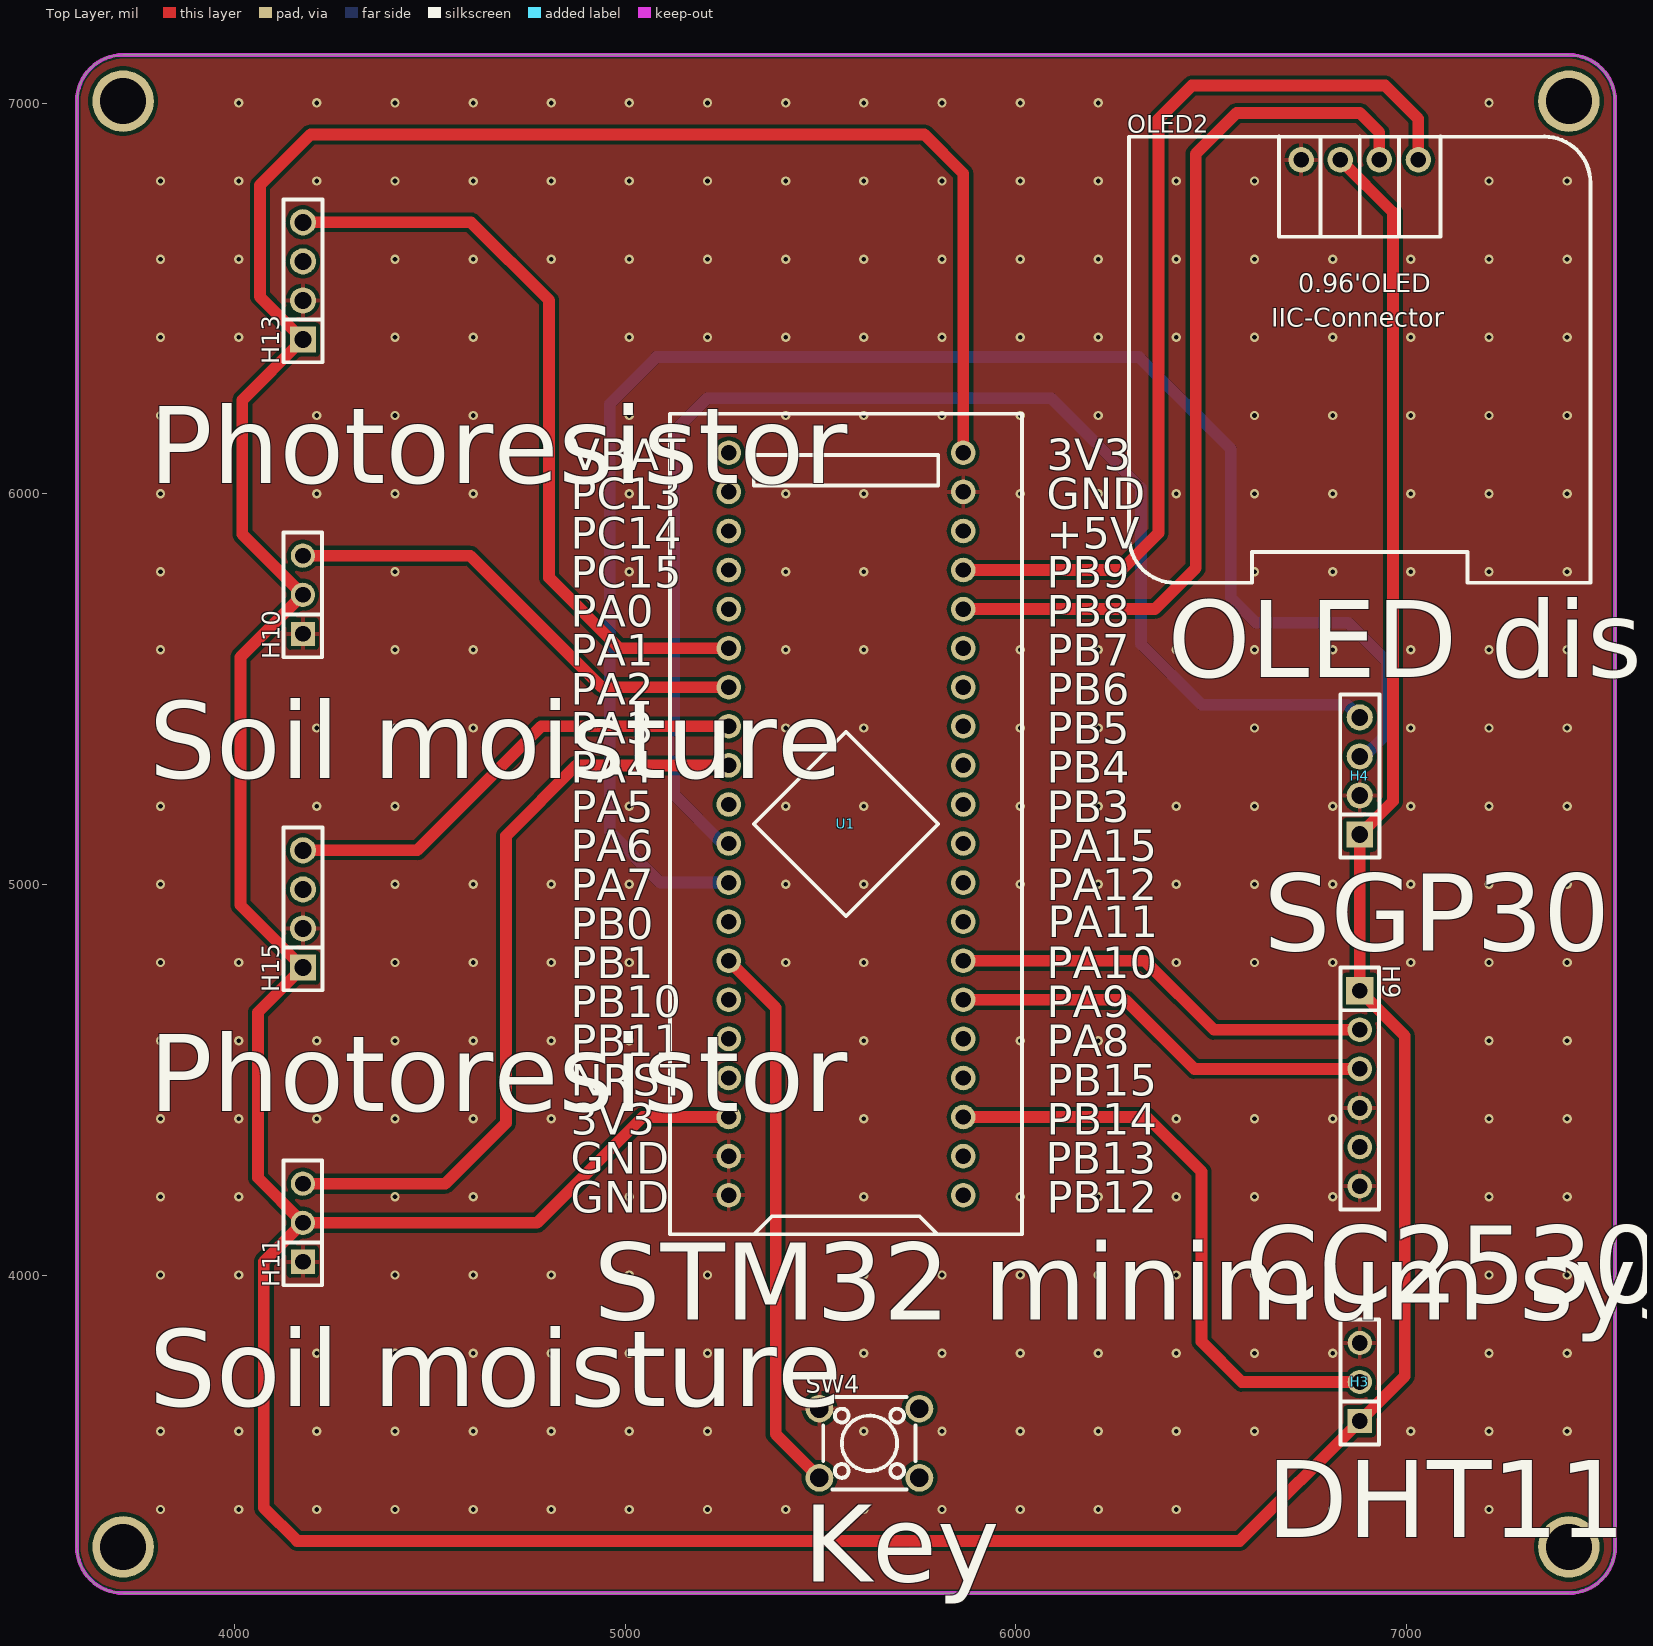
[diagram p0: Top Layer view]
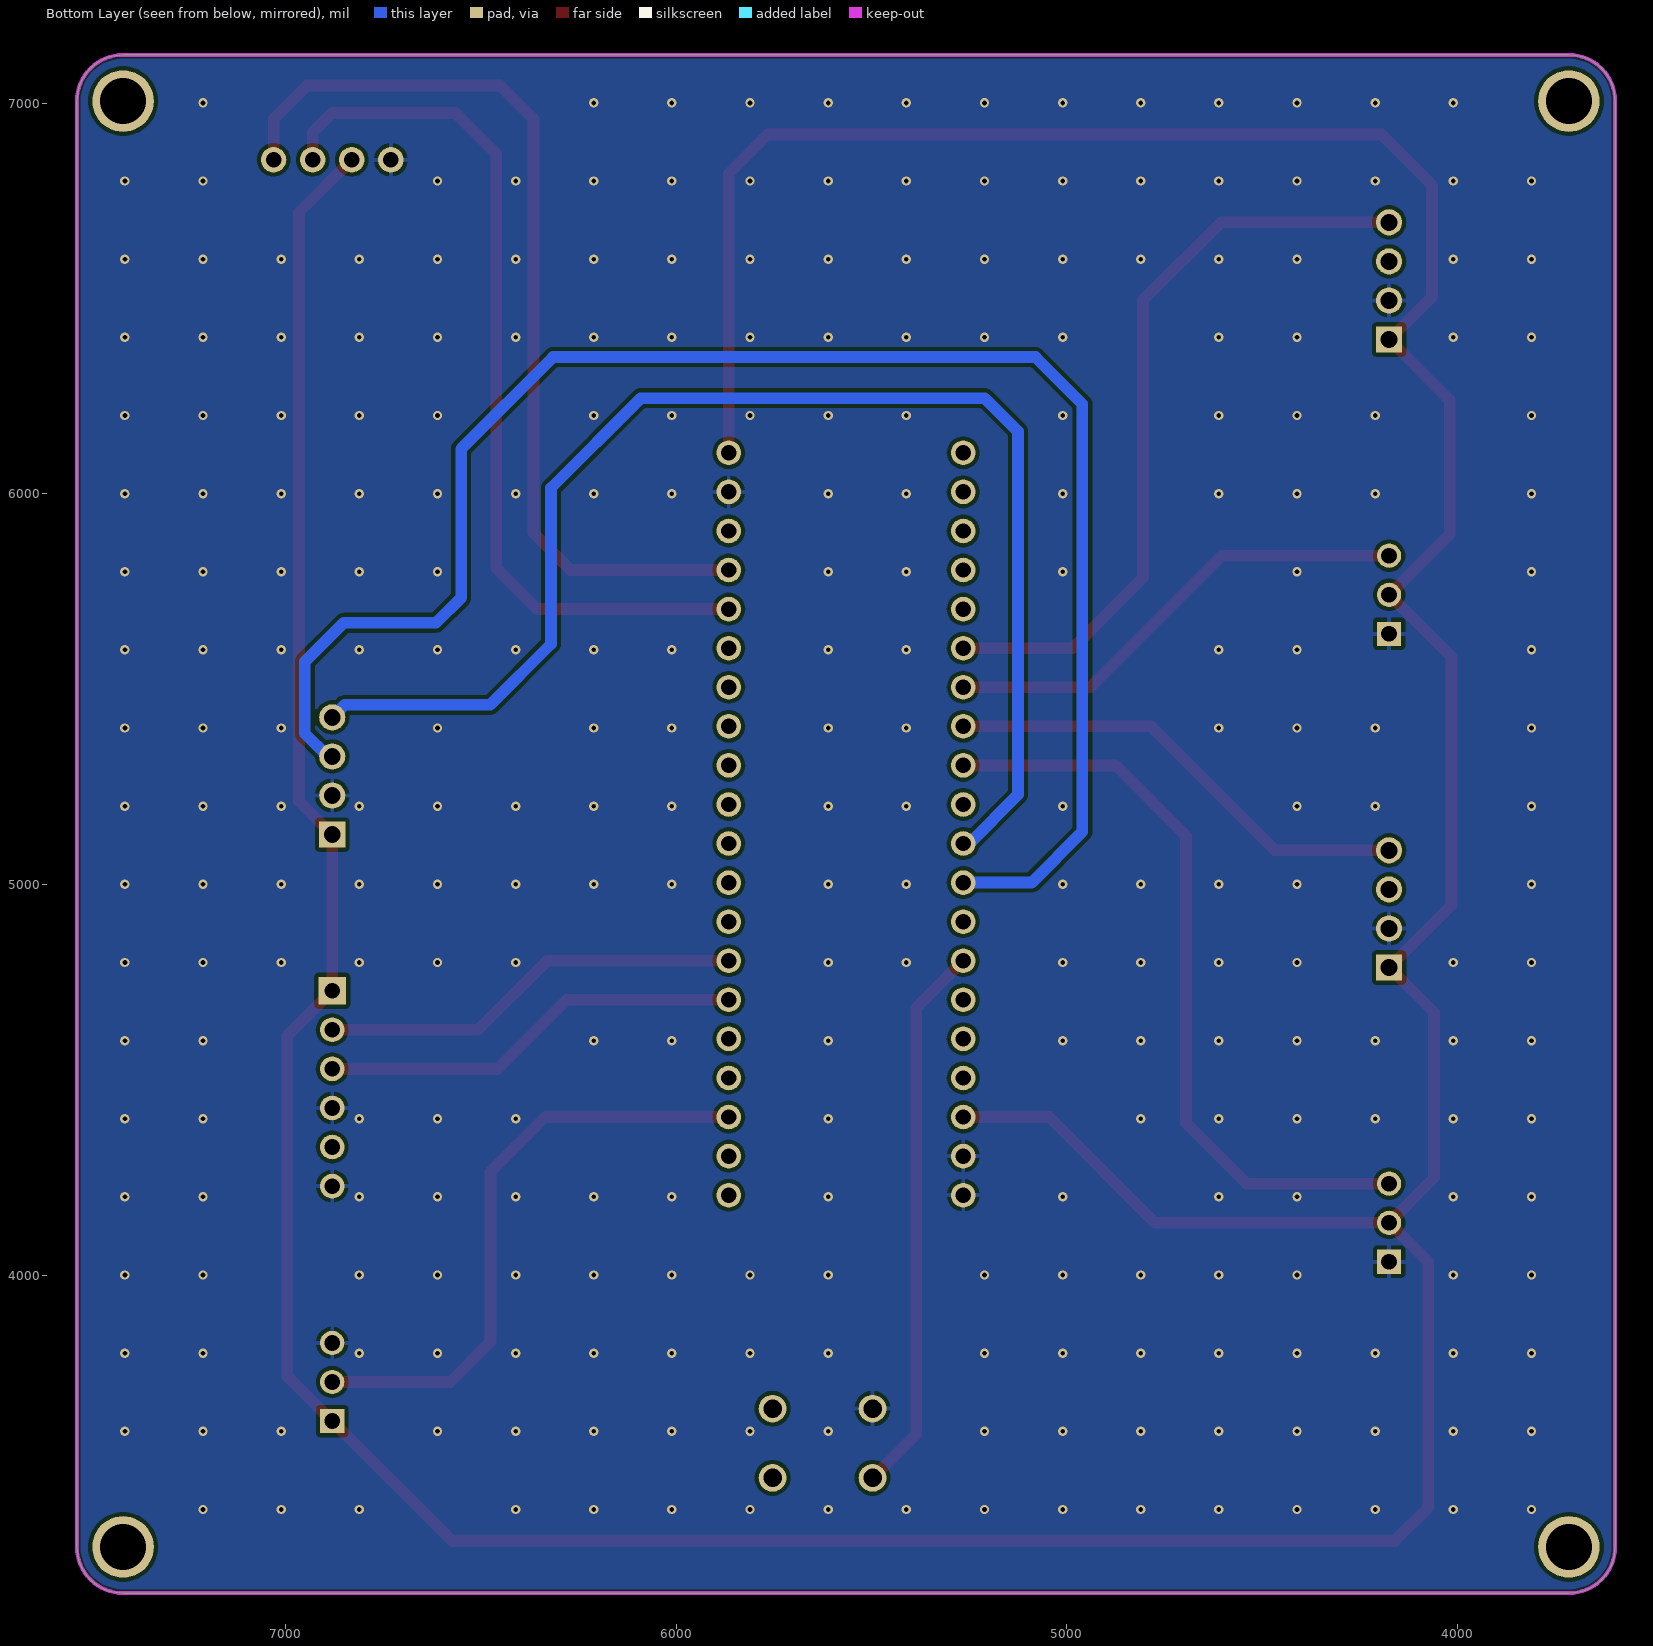
[diagram p1: Bottom Layer view, seen from below]
# Altium PCB MISC52023.pcbdoc
Units mil, origin at the board's own origin, x right, y up, seen from the top; angles counter-clockwise.
Board outline 3937.01 x 3937.01 mil, 2 copper layers (Top Layer, Bottom Layer), stack 62.206 mil thick; 10 components, 37 nets, 79 pads, 277 vias.

## Layer stack, top to bottom
Top Solder Mask Layer: solder mask 0.394, Dk 3.3
Top Layer: signal copper 1.379
Dielectric1: surface 59.449, FR4, Dk 4.5
Bottom Layer: signal copper 1.378
Bottom Solder Mask Layer: solder mask 0.394, Dk 3.3

## Board outline
3714.61,7123.5 ccw(c3714.61,7005.39) 3596.5,7005.39 3596.5,3304.61 ccw(c3714.61,3304.61) 3714.61,3186.5 7415.39,3186.5 ccw(c7415.39,3304.61) 7533.5,3304.61 7533.5,7005.39 ccw(c7415.39,7005.39) 7415.39,7123.5 3714.61,7123.5

## Design rules (kind name [scope] priority, off if disabled: settings)
BoardOutlineClearance copperThickness2oz_1 [All] p2 off: genericclearance=7.99 ignorepadtopadclearanceinfootprint=FALSE except(0: Arc-SplitContinuation Track-SplitContinuation SMDPad-SplitContinuation THPad-SplitContinuation Via-SplitContinuation Fill-SplitContinuation Region-SplitContinuation Poly-SplitContinuation Text-SplitContinuation Hole-SplitContinuation; 5.98: Arc-CutoutEdge Track-CutoutEdge SMDPad-CutoutEdge THPad-CutoutEdge Via-CutoutEdge Text-CutoutEdge; 6.9: Hole-OutlineEdge Hole-CutoutEdge; 10: Poly-OutlineEdge Poly-CutoutEdge; 11.81: Arc-OutlineEdge Track-OutlineEdge SMDPad-OutlineEdge THPad-OutlineEdge Via-OutlineEdge Fill-OutlineEdge Region-OutlineEdge Text-OutlineEdge Fill-CutoutEdge Region-CutoutEdge)
BoardOutlineClearance Plane_innerPlane_1 [All] p4 off: genericclearance=4.02 ignorepadtopadclearanceinfootprint=FALSE except(0: Arc-SplitContinuation Track-SplitContinuation SMDPad-SplitContinuation THPad-SplitContinuation Via-SplitContinuation Fill-SplitContinuation Region-SplitContinuation Poly-SplitContinuation Text-SplitContinuation Hole-SplitContinuation; 5.98: Arc-CutoutEdge Track-CutoutEdge SMDPad-CutoutEdge THPad-CutoutEdge Via-CutoutEdge Text-CutoutEdge; 6.9: Hole-OutlineEdge Hole-CutoutEdge; 10: Poly-OutlineEdge Poly-CutoutEdge; 11.81: Arc-OutlineEdge Track-OutlineEdge SMDPad-OutlineEdge THPad-OutlineEdge Via-OutlineEdge Fill-OutlineEdge Region-OutlineEdge Text-OutlineEdge Fill-CutoutEdge Region-CutoutEdge)
BoardOutlineClearance Copper_copperRegion_1 [All] p6 off: genericclearance=4.02 ignorepadtopadclearanceinfootprint=FALSE except(0: Arc-SplitContinuation Track-SplitContinuation SMDPad-SplitContinuation THPad-SplitContinuation Via-SplitContinuation Fill-SplitContinuation Region-SplitContinuation Poly-SplitContinuation Text-SplitContinuation Hole-SplitContinuation; 5.98: Arc-CutoutEdge Track-CutoutEdge SMDPad-CutoutEdge THPad-CutoutEdge Via-CutoutEdge Text-CutoutEdge; 6.9: Hole-OutlineEdge Hole-CutoutEdge; 10: Poly-OutlineEdge Poly-CutoutEdge; 11.81: Arc-OutlineEdge Track-OutlineEdge SMDPad-OutlineEdge THPad-OutlineEdge Via-OutlineEdge Fill-OutlineEdge Region-OutlineEdge Text-OutlineEdge Fill-CutoutEdge Region-CutoutEdge)
BoardOutlineClearance Copper_copperRegion_copperThickness1oz_1 [All] p8 off: genericclearance=4.02 ignorepadtopadclearanceinfootprint=FALSE except(0: Arc-SplitContinuation Track-SplitContinuation SMDPad-SplitContinuation THPad-SplitContinuation Via-SplitContinuation Fill-SplitContinuation Region-SplitContinuation Poly-SplitContinuation Text-SplitContinuation Hole-SplitContinuation; 5.98: Arc-CutoutEdge Track-CutoutEdge SMDPad-CutoutEdge THPad-CutoutEdge Via-CutoutEdge Text-CutoutEdge; 6.9: Hole-OutlineEdge Hole-CutoutEdge; 10: Poly-OutlineEdge Poly-CutoutEdge; 11.81: Arc-OutlineEdge Track-OutlineEdge SMDPad-OutlineEdge THPad-OutlineEdge Via-OutlineEdge Fill-OutlineEdge Region-OutlineEdge Text-OutlineEdge Fill-CutoutEdge Region-CutoutEdge)
BoardOutlineClearance Copper_copperRegion_Copper_copperRegion_1 [All] p10 off: genericclearance=4.02 ignorepadtopadclearanceinfootprint=FALSE except(0: Arc-SplitContinuation Track-SplitContinuation SMDPad-SplitContinuation THPad-SplitContinuation Via-SplitContinuation Fill-SplitContinuation Region-SplitContinuation Poly-SplitContinuation Text-SplitContinuation Hole-SplitContinuation; 5.98: Arc-CutoutEdge Track-CutoutEdge SMDPad-CutoutEdge THPad-CutoutEdge Via-CutoutEdge Text-CutoutEdge; 6.9: Hole-OutlineEdge Hole-CutoutEdge; 10: Poly-OutlineEdge Poly-CutoutEdge; 11.81: Arc-OutlineEdge Track-OutlineEdge SMDPad-OutlineEdge THPad-OutlineEdge Via-OutlineEdge Fill-OutlineEdge Region-OutlineEdge Text-OutlineEdge Fill-CutoutEdge Region-CutoutEdge)
BoardOutlineClearance copperThickness1oz_1 [All] p12: genericclearance=4.02 ignorepadtopadclearanceinfootprint=FALSE except(0: Arc-SplitContinuation Track-SplitContinuation SMDPad-SplitContinuation THPad-SplitContinuation Via-SplitContinuation Fill-SplitContinuation Region-SplitContinuation Poly-SplitContinuation Text-SplitContinuation Hole-SplitContinuation; 5.98: Arc-CutoutEdge Track-CutoutEdge SMDPad-CutoutEdge THPad-CutoutEdge Via-CutoutEdge Text-CutoutEdge; 6.9: Hole-OutlineEdge Hole-CutoutEdge; 10: Poly-OutlineEdge Poly-CutoutEdge; 11.81: Arc-OutlineEdge Track-OutlineEdge SMDPad-OutlineEdge THPad-OutlineEdge Via-OutlineEdge Fill-OutlineEdge Region-OutlineEdge Text-OutlineEdge Fill-CutoutEdge Region-CutoutEdge)
Clearance copperThickness2oz [All] p1 off: gap=7.99 ignorepadtopadclearanceinfootprint=FALSE except(5.98: SMDPad-Track SMDPad-SMDPad THPad-Track SMDPad-THPad THPad-THPad Track-Via SMDPad-Via THPad-Via Via-Via Fill-SMDPad Region-SMDPad Fill-THPad Region-THPad Fill-Via Region-Via Fill-Fill Fill-Region Region-Region Arc-Track Arc-SMDPad Arc-THPad Arc-Via Fill-Arc Region-Arc Arc-Arc Text-Track SMDPad-Text Text-THPad Text-Via Fill-Text Region-Text Arc-Text Text-Text; 6.9: Hole-Track Hole-SMDPad Hole-THPad Hole-Via Fill-Hole Region-Hole Hole-Arc Hole-Text; 10: Poly-Track Poly-SMDPad Poly-THPad Poly-Via Poly-Fill Poly-Region Poly-Poly Poly-Arc Poly-Text Poly-Hole; 11.81: Fill-Track Region-Track)
Clearance Plane_innerPlane [All] p3 off: gap=4.02 ignorepadtopadclearanceinfootprint=FALSE except(5.98: SMDPad-Track SMDPad-SMDPad THPad-Track SMDPad-THPad THPad-THPad Track-Via SMDPad-Via THPad-Via Via-Via Fill-SMDPad Region-SMDPad Fill-THPad Region-THPad Fill-Via Region-Via Fill-Fill Fill-Region Region-Region Arc-Track Arc-SMDPad Arc-THPad Arc-Via Fill-Arc Region-Arc Arc-Arc Text-Track SMDPad-Text Text-THPad Text-Via Fill-Text Region-Text Arc-Text Text-Text; 6.9: Hole-Track Hole-SMDPad Hole-THPad Hole-Via Fill-Hole Region-Hole Hole-Arc Hole-Text; 10: Poly-Track Poly-SMDPad Poly-THPad Poly-Via Poly-Fill Poly-Region Poly-Poly Poly-Arc Poly-Text Poly-Hole; 11.81: Fill-Track Region-Track)
Clearance Copper_copperRegion [All] p5 off: gap=4.02 ignorepadtopadclearanceinfootprint=FALSE except(5.98: SMDPad-Track SMDPad-SMDPad THPad-Track SMDPad-THPad THPad-THPad Track-Via SMDPad-Via THPad-Via Via-Via Fill-SMDPad Region-SMDPad Fill-THPad Region-THPad Fill-Via Region-Via Fill-Fill Fill-Region Region-Region Arc-Track Arc-SMDPad Arc-THPad Arc-Via Fill-Arc Region-Arc Arc-Arc Text-Track SMDPad-Text Text-THPad Text-Via Fill-Text Region-Text Arc-Text Text-Text; 6.9: Hole-Track Hole-SMDPad Hole-THPad Hole-Via Fill-Hole Region-Hole Hole-Arc Hole-Text; 10: Poly-Track Poly-SMDPad Poly-THPad Poly-Via Poly-Fill Poly-Region Poly-Poly Poly-Arc Poly-Text Poly-Hole; 11.81: Fill-Track Region-Track)
Clearance Copper_copperRegion_copperThickness1oz [All] p7 off: gap=4.02 ignorepadtopadclearanceinfootprint=FALSE except(5.98: SMDPad-Track SMDPad-SMDPad THPad-Track SMDPad-THPad THPad-THPad Track-Via SMDPad-Via THPad-Via Via-Via Fill-SMDPad Region-SMDPad Fill-THPad Region-THPad Fill-Via Region-Via Fill-Fill Fill-Region Region-Region Arc-Track Arc-SMDPad Arc-THPad Arc-Via Fill-Arc Region-Arc Arc-Arc Text-Track SMDPad-Text Text-THPad Text-Via Fill-Text Region-Text Arc-Text Text-Text; 6.9: Hole-Track Hole-SMDPad Hole-THPad Hole-Via Fill-Hole Region-Hole Hole-Arc Hole-Text; 10: Poly-Track Poly-SMDPad Poly-THPad Poly-Via Poly-Fill Poly-Region Poly-Poly Poly-Arc Poly-Text Poly-Hole; 11.81: Fill-Track Region-Track)
Clearance Copper_copperRegion_Copper_copperRegion [All] p9 off: gap=4.02 ignorepadtopadclearanceinfootprint=FALSE except(5.98: SMDPad-Track SMDPad-SMDPad THPad-Track SMDPad-THPad THPad-THPad Track-Via SMDPad-Via THPad-Via Via-Via Fill-SMDPad Region-SMDPad Fill-THPad Region-THPad Fill-Via Region-Via Fill-Fill Fill-Region Region-Region Arc-Track Arc-SMDPad Arc-THPad Arc-Via Fill-Arc Region-Arc Arc-Arc Text-Track SMDPad-Text Text-THPad Text-Via Fill-Text Region-Text Arc-Text Text-Text; 6.9: Hole-Track Hole-SMDPad Hole-THPad Hole-Via Fill-Hole Region-Hole Hole-Arc Hole-Text; 10: Poly-Track Poly-SMDPad Poly-THPad Poly-Via Poly-Fill Poly-Region Poly-Poly Poly-Arc Poly-Text Poly-Hole; 11.81: Fill-Track Region-Track)
Clearance copperThickness1oz [All] p11: gap=4.02 ignorepadtopadclearanceinfootprint=FALSE except(5.98: SMDPad-Track SMDPad-SMDPad THPad-Track SMDPad-THPad THPad-THPad Track-Via SMDPad-Via THPad-Via Via-Via Fill-SMDPad Region-SMDPad Fill-THPad Region-THPad Fill-Via Region-Via Fill-Fill Fill-Region Region-Region Arc-Track Arc-SMDPad Arc-THPad Arc-Via Fill-Arc Region-Arc Arc-Arc Text-Track SMDPad-Text Text-THPad Text-Via Fill-Text Region-Text Arc-Text Text-Text; 6.9: Hole-Track Hole-SMDPad Hole-THPad Hole-Via Fill-Hole Region-Hole Hole-Arc Hole-Text; 10: Poly-Track Poly-SMDPad Poly-THPad Poly-Via Poly-Fill Poly-Region Poly-Poly Poly-Arc Poly-Text Poly-Hole; 11.81: Fill-Track Region-Track)
DiffPairsRouting differentialPair [All] p1: maxlimit=6 minlimit=6 mostfreqgap=6 toplayer_minwidth=5 toplayer_prefwidth=10 toplayer_maxwidth=100 toplayer_mingap=6 toplayer_prefgap=6 toplayer_maxgap=6 bottomlayer_minwidth=5 bottomlayer_prefwidth=10 bottomlayer_maxwidth=100 bottomlayer_mingap=6 bottomlayer_prefgap=6 bottomlayer_maxgap=6 maxuncoupledlength=10
HoleToHoleClearance otherClearance [All] p1: gap=11.81 allowstackedmicrovias=TRUE
Length netLength [All] p1: minlimit=0 maxlimit=0
PasteMaskExpansion pasteMaskExpansion [All] p1: expansion=0
PlaneConnect innerPlane [All] p1: planeconnectstyle=Relief reliefexpansion=20 reliefentries=4 reliefconductorwidth=10 reliefairgap=10
PolygonConnect copperRegion_copperThickness1oz [All] p1 off: connectstyle=Relief reliefconductorwidth=10 reliefentries=4 polygonreliefangle="90 Angle" airgapwidth=10 via.connectstyle=Relief via.reliefconductorwidth=10 via.reliefentries=4 via.polygonreliefangle="90 Angle" via.airgapwidth=10
PolygonConnect copperRegion_Copper_copperRegion [All] p2 off: connectstyle=Relief reliefconductorwidth=10 reliefentries=4 polygonreliefangle="90 Angle" airgapwidth=10 via.connectstyle=Relief via.reliefconductorwidth=10 via.reliefentries=4 via.polygonreliefangle="90 Angle" via.airgapwidth=10
PolygonConnect copperRegion [All] p3: connectstyle=Relief reliefconductorwidth=10 reliefentries=4 polygonreliefangle="90 Angle" airgapwidth=10 via.connectstyle=Relief via.reliefconductorwidth=10 via.reliefentries=4 via.polygonreliefangle="90 Angle" via.airgapwidth=10
RoutingVias viaSize [All] p1: holewidth=12.01 width=24.02 viastyle="Through Hole" minholewidth=11.81 minwidth=19.68 maxholewidth=248.03 maxwidth=393.7
SolderMaskExpansion solderMaskExpansion [IsVia] p1: expansion=-1000 istentingtop=TRUE
SolderMaskExpansion solderMaskExpansion [All] p2: expansion=2 istentingtop=FALSE
Width copperThickness2oz_2 [All] p1 off: maxlimit=100 minlimit=8 preferedwidth=10
Width copperThickness1oz_2 [All] p2: maxlimit=100 minlimit=5 preferedwidth=10

## Components (designator, comment, footprint, x,y, rotation, side; value= is the part's Value field where it differs from the comment)
H3 "" HDR-TH_3P-P2.54-V-F 6880,3726.86 r90 top
H4 "" HDR-TH_4P-P2.54-V-F 6880,5277.96 r90 top
H9 "" HDR-TH_6P-P2.54-V-F 6880,4478.2 r270 top
H10 "" HDR-TH_3P-P2.54-V-F 4175,5741.64 r90 top
H11 "" HDR-TH_3P-P2.54-V-F 4175,4134.33 r90 top
H13 "" HDR-TH_4P-P2.54-V-F 4175,6545 r90 top
H15 "" HDR-TH_4P-P2.54-V-F 4175,4937.69 r90 top
OLED2 "" 0.96OLED_4P 6880,6855 r0 top
SW4 "" SW-TH_4P-L6.0-W6.0-P4.50-LS6.5 5625,3570 r0 top
U1 "STM32F103C8T6-Card" CONN-TH_L53.3-W22.9_STM32F103C8T6-CARD 5565,5155 r90 top

## Footprints (in the part's own frame and the unit in brackets; to place one, negate y for a bottom-side part, rotate by r counter-clockwise, add the part's x,y. Pads: shape width x height; smd on the part's side, far side on the other; paste and mask are expansions set on the pad)
0.96OLED_4P [mm]
  round 1.65 hole 1 copper offset 0,0: 1(-3.81,-0.001) 2(-1.27,0.002) 3(1.27,0.002) 4(3.81,0.002)
  silkscreen extent -15,-27.5 15,1.5
CONN-TH_L53.3-W22.9_STM32F103C8T6-CARD [mm]
  round 1.6 hole 1: 1(-24.13,-7.62) 2(-21.59,-7.62) 3(-19.05,-7.62) 4(-16.51,-7.62) 5(-13.97,-7.62) 6(-11.43,-7.62) 7(-8.89,-7.62) 8(-6.35,-7.62) 9(-3.81,-7.62) 10(-1.27,-7.62) 11(1.27,-7.62) 12(3.81,-7.62) 13(6.35,-7.62) 14(8.89,-7.62) 15(11.43,-7.62) 16(13.97,-7.62) 17(16.51,-7.62) 18(19.05,-7.62) 19(21.59,-7.62) 20(24.13,-7.62) 21(24.13,7.62) 22(21.59,7.62) 23(19.05,7.62) 24(16.51,7.62) 25(13.97,7.62) 26(11.43,7.62) 27(8.89,7.62) 28(6.35,7.62) 29(3.81,7.62) 30(1.27,7.62) 31(-1.27,7.62) 32(-3.81,7.62) 33(-6.35,7.62) 34(-8.89,7.62) 35(-11.43,7.62) 36(-13.97,7.62) 37(-16.51,7.62) 38(-19.05,7.62) 39(-21.59,7.62) 40(-24.13,7.62)
  silkscreen extent -26.67,-11.43 26.67,11.43
HDR-TH_3P-P2.54-V-F [mil]
  rect 62x62 hole 40.16: 1(-100,0)
  round 62 hole 40.16: 2(0,0) 3(100,0)
  silkscreen extent -160,-49 160,49
HDR-TH_4P-P2.54-V-F [mm]
  rect 1.7x1.7 hole 1.1: 1(-3.81,0)
  round 1.7 hole 1.1: 2(-1.27,0) 3(1.27,0) 4(3.81,0)
  silkscreen extent -5.29,-1.27 5.29,1.27
HDR-TH_6P-P2.54-V-F [mm]
  rect 1.8x1.8 hole 1.02: 1(-6.35,0)
  round 1.6 hole 1.02: 2(-3.81,0) 3(-1.27,0) 4(1.27,0) 5(3.81,0) 6(6.35,0)
  silkscreen extent -7.87,-1.25 7.87,1.25
SW-TH_4P-L6.0-W6.0-P4.50-LS6.5 [mm]
  round 1.8 hole 1.2: 1(-3.25,2.25) 2(3.25,2.25) 3(-3.25,-2.25) 4(3.25,-2.25)
  silkscreen extent -3,-3 3,3

## Free pads (board coordinates)
  round 157.48 hole 118.11: 1(3714.61,7005.39) 1(3714.61,3304.61) 1(7415.39,7005.39) 1(7415.39,3304.61)

## Via types
v1: diameter 24.02, hole 12, Top Layer to Bottom Layer, 277 vias

## Nets (pads, with @x,y where several pads share a name; then routed paths per layer and width w, separated by ;. In a path a pad name is that pad's centre, name@x,y a point inside that pad or via, vN(x,y) a via of type N, cw(c..) or ccw(c..) an arc to the next point about the centre after c; other vN are vias at no path point)
+5V: U1.18
GND: H3.3 H4.2 H9.4 H9.6 H10.1 H11.1 H13.2 H15.2 OLED2.1 SW4.1 U1.19 U1.39 U1.40
  other v1: 3810.6,3400.6 4010.6,3400.6 4210.6,3400.6 4410.6,3400.6 4610.6,3400.6 4810.6,3400.6 5010.6,3400.6 5210.6,3400.6 5410.6,3400.6 5610.6,3400.6 5810.6,3400.6 6010.6,3400.6 6210.6,3400.6 6410.6,3400.6 6810.6,3400.6 7010.6,3400.6 7210.6,3400.6 3810.6,3600.6 4010.6,3600.6 4210.6,3600.6 4410.6,3600.6 4610.6,3600.6 4810.6,3600.6 5010.6,3600.6 5210.6,3600.6 5610.6,3600.6 5810.6,3600.6 6010.6,3600.6 6210.6,3600.6 6410.6,3600.6 6610.6,3600.6 7010.6,3600.6 7210.6,3600.6 7410.6,3600.6 3810.6,3800.6 4010.6,3800.6 4210.6,3800.6 4410.6,3800.6 4610.6,3800.6 4810.6,3800.6 5010.6,3800.6 5210.6,3800.6 5610.6,3800.6 5810.6,3800.6 6010.6,3800.6 6210.6,3800.6 6410.6,3800.6 6610.6,3800.6 6810.6,3800.6 7210.6,3800.6 7410.6,3800.6 3810.6,4000.6 4010.6,4000.6 4410.6,4000.6 4610.6,4000.6 4810.6,4000.6 5010.6,4000.6 5210.6,4000.6 5610.6,4000.6 5810.6,4000.6 6010.6,4000.6 6210.6,4000.6 6410.6,4000.6 6610.6,4000.6 6810.6,4000.6 7210.6,4000.6 7410.6,4000.6 3810.6,4200.6 4010.6,4200.6 4410.6,4200.6 4610.6,4200.6 5010.6,4200.6 5610.6,4200.6 6010.6,4200.6 6210.6,4200.6 6410.6,4200.6 6610.6,4200.6 6810.6,4200.6 7210.6,4200.6 7410.6,4200.6 3810.6,4400.6 4010.6,4400.6 4210.6,4400.6 4410.6,4400.6 4610.6,4400.6 4810.6,4400.6 5610.6,4400.6 6410.6,4400.6 6610.6,4400.6 6810.6,4400.6 7210.6,4400.6 7410.6,4400.6 3810.6,4600.6 4010.6,4600.6 4210.6,4600.6 4410.6,4600.6 4610.6,4600.6 4810.6,4600.6 5010.6,4600.6 5610.6,4600.6 6010.6,4600.6 6210.6,4600.6 7210.6,4600.6 7410.6,4600.6 3810.6,4800.6 4010.6,4800.6 4410.6,4800.6 4610.6,4800.6 4810.6,4800.6 5010.6,4800.6 5410.6,4800.6 5610.6,4800.6 6410.6,4800.6 6610.6,4800.6 6810.6,4800.6 7010.6,4800.6 7210.6,4800.6 7410.6,4800.6 3810.6,5000.6 4410.6,5000.6 4610.6,5000.6 4810.6,5000.6 5010.6,5000.6 5410.6,5000.6 5610.6,5000.6 6010.6,5000.6 6210.6,5000.6 6410.6,5000.6 6610.6,5000.6 6810.6,5000.6 7010.6,5000.6 7210.6,5000.6 7410.6,5000.6 3810.6,5200.6 4210.6,5200.6 4410.6,5200.6 5010.6,5200.6 5410.6,5200.6 5610.6,5200.6 6010.6,5200.6 6210.6,5200.6 6410.6,5200.6 6610.6,5200.6 6810.6,5200.6 7010.6,5200.6 7210.6,5200.6 7410.6,5200.6 3810.6,5400.6 4210.6,5400.6 4410.6,5400.6 4610.6,5400.6 5410.6,5400.6 5610.6,5400.6 6010.6,5400.6 6210.6,5400.6 6610.6,5400.6 7010.6,5400.6 7210.6,5400.6 7410.6,5400.6 3810.6,5600.6 4410.6,5600.6 4610.6,5600.6 5410.6,5600.6 5610.6,5600.6 6010.6,5600.6 6210.6,5600.6 6410.6,5600.6 6610.6,5600.6 6810.6,5600.6 7010.6,5600.6 7210.6,5600.6 7410.6,5600.6 3810.6,5800.6 4410.6,5800.6 5010.6,5800.6 5410.6,5800.6 5610.6,5800.6 6610.6,5800.6 6810.6,5800.6 7010.6,5800.6 7210.6,5800.6 7410.6,5800.6 3810.6,6000.6 4210.6,6000.6 4410.6,6000.6 4610.6,6000.6 5010.6,6000.6 5410.6,6000.6 5610.6,6000.6 6010.6,6000.6 6210.6,6000.6 6410.6,6000.6 6610.6,6000.6 6810.6,6000.6 7010.6,6000.6 7210.6,6000.6 7410.6,6000.6 3810.6,6200.6 4210.6,6200.6 4410.6,6200.6 4610.6,6200.6 5010.6,6200.6 5410.6,6200.6 5610.6,6200.6 5810.6,6200.6 6010.6,6200.6 6210.6,6200.6 6610.6,6200.6 6810.6,6200.6 7010.6,6200.6 7210.6,6200.6 7410.6,6200.6 3810.6,6400.6 4010.6,6400.6 4410.6,6400.6 4610.6,6400.6 5010.6,6400.6 5210.6,6400.6 5410.6,6400.6 5610.6,6400.6 5810.6,6400.6 6010.6,6400.6 6210.6,6400.6 6410.6,6400.6 6610.6,6400.6 6810.6,6400.6 7010.6,6400.6 7210.6,6400.6 7410.6,6400.6 3810.6,6600.6 4010.6,6600.6 4410.6,6600.6 4610.6,6600.6 4810.6,6600.6 5010.6,6600.6 5210.6,6600.6 5410.6,6600.6 5610.6,6600.6 5810.6,6600.6 6010.6,6600.6 6210.6,6600.6 6410.6,6600.6 6610.6,6600.6 6810.6,6600.6 7010.6,6600.6 7210.6,6600.6 7410.6,6600.6 3810.6,6800.6 4010.6,6800.6 4210.6,6800.6 4410.6,6800.6 4610.6,6800.6 4810.6,6800.6 5010.6,6800.6 5210.6,6800.6 5410.6,6800.6 5610.6,6800.6 5810.6,6800.6 6010.6,6800.6 6210.6,6800.6 6410.6,6800.6 6610.6,6800.6 7210.6,6800.6 7410.6,6800.6 4010.6,7000.6 4210.6,7000.6 4410.6,7000.6 4610.6,7000.6 4810.6,7000.6 5010.6,7000.6 5210.6,7000.6 5410.6,7000.6 5610.6,7000.6 5810.6,7000.6 6010.6,7000.6 6210.6,7000.6 7210.6,7000.6
NRST: U1.37
PA0: U1.25
PA1: H13.4 U1.26 | length 1957.4
  Top Layer w30: H13.4 4605,6695 4805,6495 4805,5785 4985,5605 U1.26
PA2: H10.3 U1.27 | length 1229.4
  Top Layer w30: H10.3 4603.36,5841.64 4940,5505 U1.27
PA3: H15.4 U1.28 | length 1221.4
  Top Layer w30: H15.4 4467.69,5087.69 4785,5405 U1.28
PA4: H11.3 U1.29 | length 1964
  Top Layer w30: H11.3 4539.33,4234.33 4695,4390 4695,5125 4875,5305 U1.29
PA5: U1.30
PA6: H4.4 U1.31 | length 3484.3
  Bottom Layer w30: U1.31 5250,5105 5125,5230 5125,6160 5210,6245 6090,6245 6320,6015 6320,5615.65 6475.65,5460 6847.95,5460 H4.4
PA7: H4.3 U1.32 | length 4317.2
  Bottom Layer w30: U1.32 5090,5005 4960,5135 4960,6230 5080,6350 6315,6350 6550,6115 6550,5734.43 6614.43,5670 6850,5670 6950,5570 6950,5386.71 6891.25,5327.96 H4.3
PA8: U1.5
PA9: H9.3 U1.6 | length 1088.2
  Top Layer w30: U1.6 6280,4705 6456.8,4528.2 H9.3
PA10: H9.2 U1.7 | length 1088.2
  Top Layer w30: U1.7 6330,4805 6506.8,4628.2 H9.2
PA11: U1.8
PA12: U1.9
PA15: U1.10
PB0: U1.33
PB1: SW4.3 U1.34 | length 1419.7
  Top Layer w30: U1.34 5385,4685 5385,3593.47 SW4.3
PB3: U1.11
PB4: U1.12
PB5: U1.13
PB6: U1.14
PB7: U1.15
PB8: OLED2.3 U1.16 | length 2302.6
  Top Layer w30: U1.16 6355,5705 6460,5810 6460,6870 6565,6975 6880,6975 6930,6925 OLED2.3@6930,6855.05
PB9: OLED2.4 U1.17 | length 2439.7
  Top Layer w30: U1.17 6270,5805 6365,5900 6365,6960 6450,7045 6945,7045 7030,6960 OLED2.4@7030,6855.05
PB10: U1.35
PB11: U1.36
PB12: U1.1
PB13: U1.2
PB14: H3.2 U1.3 | length 1550.7
  Top Layer w30: U1.3 6335,4405 6475,4265 6475,3830 6578.14,3726.86 H3.2
PB15: U1.4
PC13: U1.22
PC14: U1.23
PC15: U1.24
VBAT: U1.21
VCC: H3.1 H4.1 H9.1 H10.2 H11.2 H13.1 H15.1 OLED2.2 U1.20 U1.38 | length 14022.5
  Top Layer w30: U1.38 5045,4405 4774.33,4134.33 H11.2 ; U1.20 5865,6820 5765,6920 4195,6920 4065,6790 4065,6505 H13.1 4020,6240 4020,5896.64 H10.2 4015,5581.64 4015,4947.69 H15.1 4060,4672.69 4060,4249.33 H11.2 ; OLED2.2@6830,6855.05 6965,6720.05 6965,5212.96 H4.1 H9.1 6995,4613.19 6995,3741.86 H3.1 6573.14,3320 4160,3320 4075,3405 4075,4034.33 H11.2
pads on no net: H9.5 H13.3 H15.3 SW4.2 SW4.4

## Polygon pours and split planes (outlines as drawn)
GND on Bottom Layer (solid, remove dead copper, pour order 2): 3525,7245 3525,3080 7700,3080 7700,7245
GND on Top Layer (solid, remove dead copper, pour order 2): 3000,7415 3000,3000 7930,3000 7930,7415

## Keep-outs
Board Outline Layer:
  the board outline again, w10

## Silkscreen, mask and mechanical layers (free items; w line width, h text height)
Top Silkscreen Layer:
  text "VBAT" at 4860.95,6060 h80
  text "3V3" at 6079.16,6060 h80
  text "Photoresistor" at 3781.86,6027.24 h196.85
  text "PC13" at 4860.95,5960 h80
  text "GND" at 6079.16,5960 h80
  text "PC14" at 4860.95,5860 h80
  text "+5V" at 6079.16,5860 h80
  text "PC15" at 4860.95,5760 h80
  text "PB9" at 6079.16,5760 h80
  text "PA0" at 4860.95,5660 h80
  text "PB8" at 6079.16,5660 h80
  text "PA1" at 4860.95,5560 h80
  text "PB7" at 6079.16,5560 h80
  text "OLED display" at 6388.02,5530.87 h196.85
  text "PA2" at 4860.95,5460 h80
  text "PB6" at 6079.16,5460 h80
  text "PA3" at 4860.95,5360 h80
  text "PB5" at 6079.16,5360 h80
  text "Soil moisture" at 3781.75,5272.31 h196.85
  text "PA4" at 4860.95,5260 h80
  text "PB4" at 6079.16,5260 h80
  text "PA5" at 4860.95,5160 h80
  text "PB3" at 6079.16,5160 h80
  text "PA6" at 4860.95,5060 h80
  text "PA15" at 6079.16,5060 h80
  text "PA7" at 4860.95,4960 h80
  text "PA12" at 6079.16,4960 h80
  text "PA11" at 6080.95,4865 h80
  text "PB0" at 4860.95,4860 h80
  text "SGP30" at 6634.83,4831.18 h196.85
  text "PB1" at 4860.95,4760 h80
  text "PA10" at 6079.16,4760 h80
  text "PB10" at 4860.95,4660 h80
  text "PA9" at 6079.16,4660 h80
  text "PB11" at 4860.95,4560 h80
  text "PA8" at 6079.16,4560 h80
  text "NRST" at 4860.95,4460 h80
  text "PB15" at 6079.16,4460 h80
  text "Photoresistor" at 3781.86,4419.93 h196.85
  text "3V3" at 4860.95,4360 h80
  text "PB14" at 6079.16,4360 h80
  text "GND" at 4860.95,4260 h80
  text "PB13" at 6075.95,4260 h80
  text "GND" at 4860.95,4160 h80
  text "PB12" at 6079.16,4160 h80
  text "CC2530" at 6587.11,3929.85 h196.85
  text "STM32 minimum system" at 4919.45,3886.57 h196.85
  text "Soil moisture" at 3781.75,3665 h196.85
  text "DHT11" at 6641.39,3330 h196.85
  text "Key" at 5455,3215 h196.85